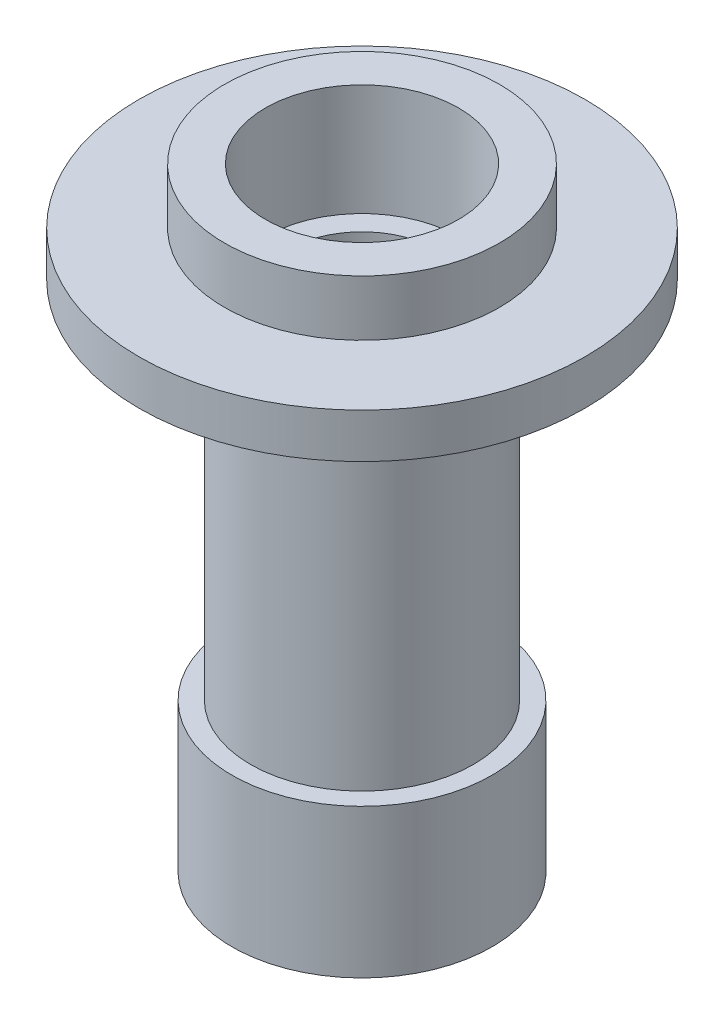
from build123d import *


with BuildPart() as part:
    # Sketch1 → Revolve1 (revolve)
    with BuildSketch(Plane.XY.offset(-440.692981355), mode=Mode.PRIVATE) as revolve1_sk:
        Polygon((551.230642584, 721.895595987), (551.230642584, 804.895595987), (556.230642584, 804.895595987), (556.230642584, 819.895595987), (581.230642584, 819.895595987), (581.230642584, 831.895595987), (558.230642584, 831.895595987), (558.230642584, 846.895595987), (547.230642584, 846.895595987), (547.230642584, 816.895595987), (541.230642584, 816.895595987), (541.230642584, 701.895595987), (547.230642584, 701.895595987), (547.230642584, 681.895595987), (556.230642584, 681.895595987), (556.230642584, 721.895595987), align=None)
    revolve(revolve1_sk.sketch.rotate(Axis((521.230642584, 846.895595987, -440.692981355), (0, -1, 0)), 270), axis=Axis((521.230642584, 846.895595987, -440.692981355), (0, -1, 0)))


solid = part.part
